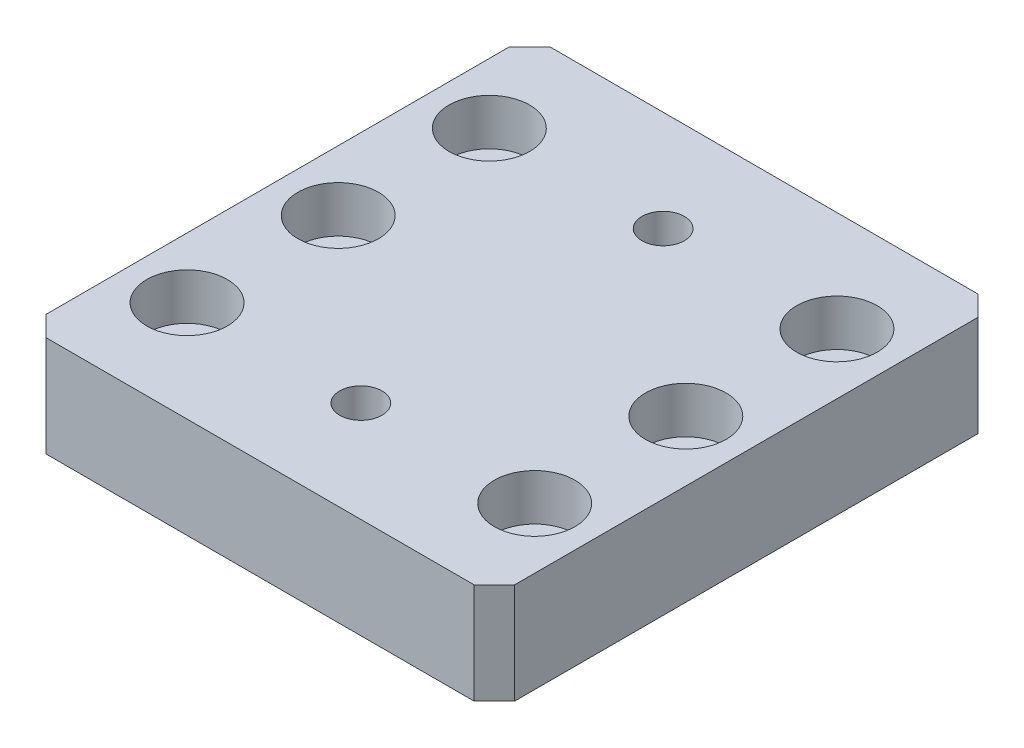
from build123d import *

# Parameters (mm, degrees)
SKETCH_1_W                = 46.5
SKETCH_1_H                = 50
EXTRUDE_1_DEPTH           = 10
HOLE_WIZARD_1_D           = 4.5
HOLE_WIZARD_1_DEPTH       = 20
HOLE_WIZARD_1_CBORE_D     = 8
HOLE_WIZARD_1_CBORE_DEPTH = 4.6
HOLE_WIZARD_1_TIP         = 1.351936393
CHAMFER_1_SIZE            = 2
HOLE_WIZARD_M5_1_D        = 4.2


with BuildPart() as part:
    # 草图1 → 凸台-拉伸1 (new body)
    with BuildSketch(Plane(origin=(0, 0, 0), x_dir=(1, 0, 0), z_dir=(0, 1, 0))):
        Rectangle(SKETCH_1_W, SKETCH_1_H)
    extrude(amount=EXTRUDE_1_DEPTH)

    # 打孔尺寸(%根据)内六角圆柱头螺钉的类型1
    with Locations(Plane(origin=(0, 10, 0), x_dir=(1, 0, 0), z_dir=(0, 1, 0))):
        with Locations((17.25, -15), (17.25, 0), (17.25, 15), (-17.25, 15), (-17.25, 0), (-17.25, -15)):
            CounterBoreHole(HOLE_WIZARD_1_D / 2, HOLE_WIZARD_1_CBORE_D / 2, HOLE_WIZARD_1_CBORE_DEPTH, depth=HOLE_WIZARD_1_DEPTH)
            with Locations((0, 0, -(HOLE_WIZARD_1_DEPTH + HOLE_WIZARD_1_TIP / 2))):  # 118° drill point
                Cone(0, HOLE_WIZARD_1_D / 2, HOLE_WIZARD_1_TIP, mode=Mode.SUBTRACT)

    # 倒角1
    chamfer_1_edges = [part.edges().sort_by_distance(p)[0] for p in [
        (23.25, 5, 25),
        (-23.25, 5, 25),
        (-23.25, 5, -25),
        (23.25, 5, -25),
    ]]
    chamfer(chamfer_1_edges, length=CHAMFER_1_SIZE)

    # M5 螺纹孔1 (through all)
    with Locations(Plane(origin=(0, 10, 0), x_dir=(1, 0, 0), z_dir=(0, 1, 0))):
        with Locations((0, 15), (0, -15)):
            Hole(HOLE_WIZARD_M5_1_D / 2)


solid = part.part
